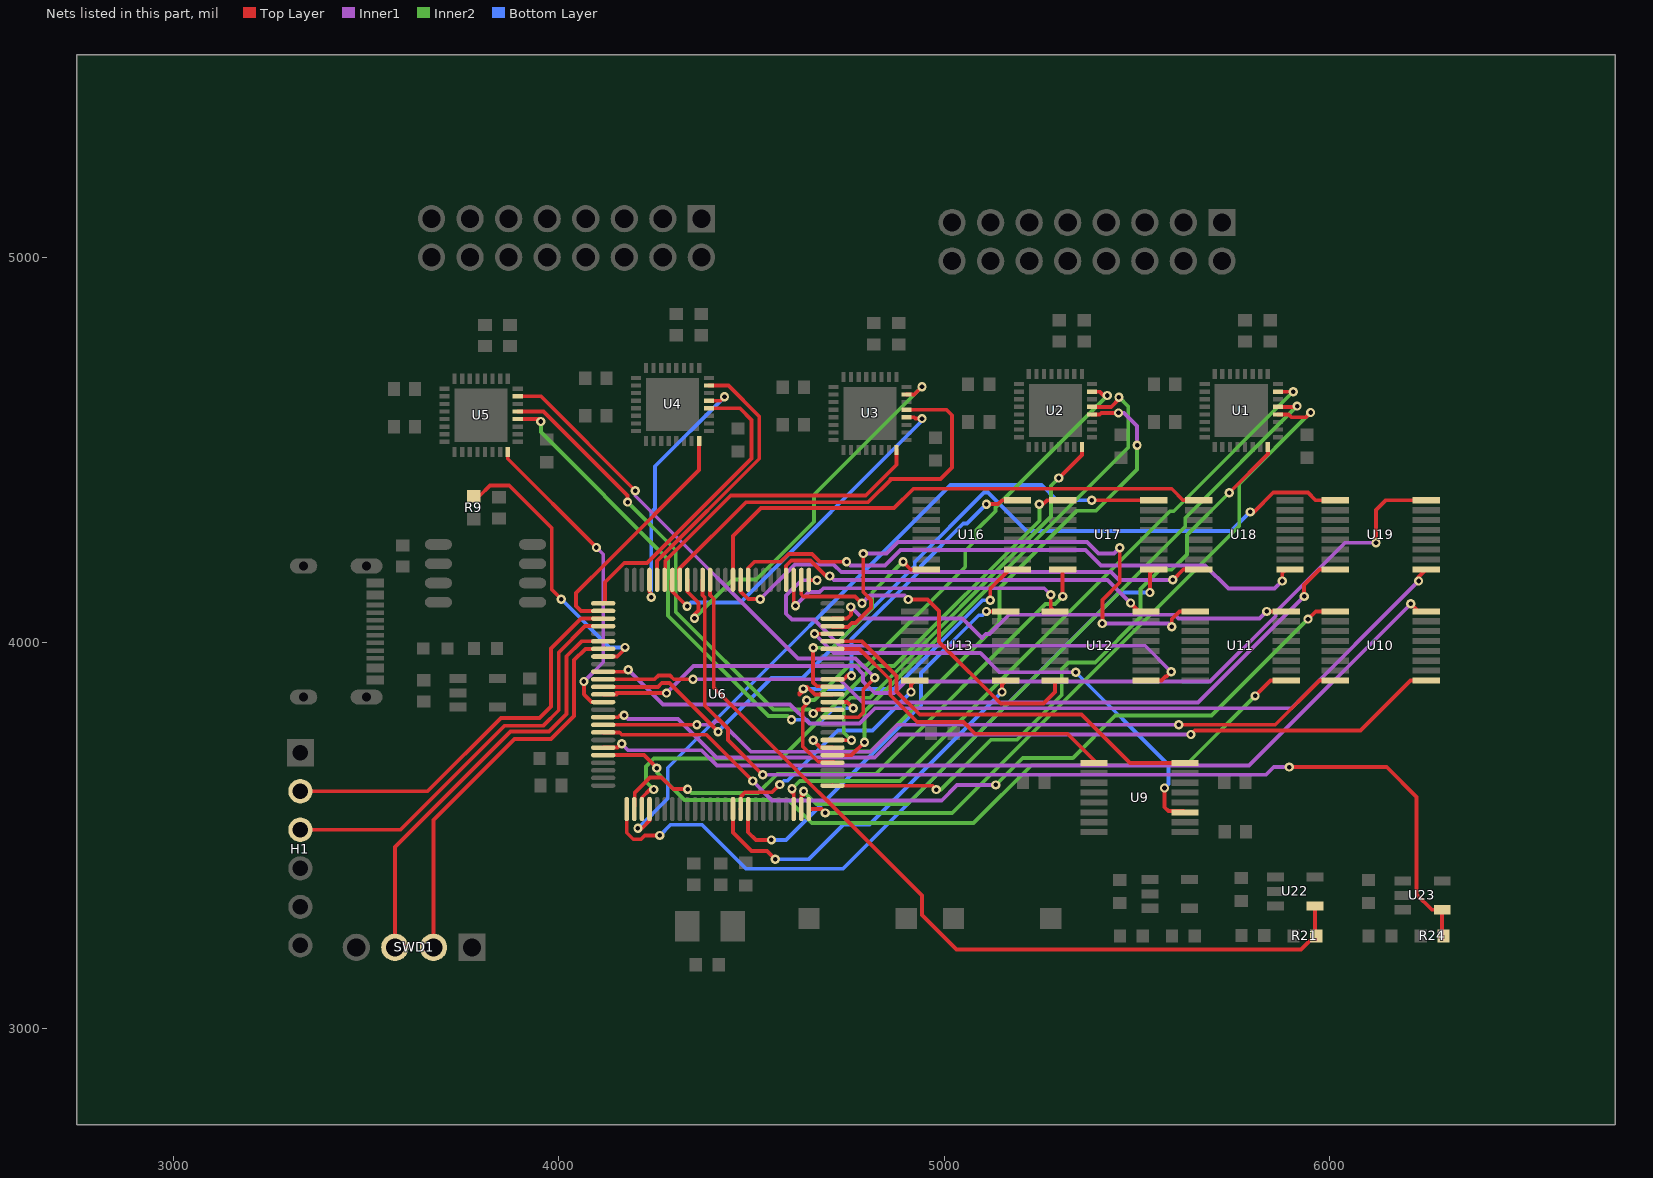
[diagram p0: the nets of this part, all layers, seen from the top]
# Altium PCB MISC49858.pcbdoc (part 3 of 3)
Units mil, origin at the board's own origin, x right, y up, seen from the top; angles counter-clockwise.
Board outline 3990 x 2775 mil, 6 copper layers (Top Layer, Inner1, Inner2, Inner3, Inner4, Bottom Layer), stack 60.565 mil thick; 79 components, 151 nets, 603 pads, 275 vias.

## Via types
v1: diameter 24.02, hole 12, Top Layer to Bottom Layer, 275 vias

## Nets (pads, with @x,y where several pads share a name; then routed paths per layer and width w, separated by ;. In a path a pad name is that pad's centre, name@x,y a point inside that pad or via, vN(x,y) a via of type N, cw(c..) or ccw(c..) an arc to the next point about the centre after c; other vN are vias at no path point) (continued)
OUT2: R21.2 U6.64 U22.4 | length 2252.9
  Top Layer w10: U6.64@4392.85,4163.23 4391.96,4162.33 4391.96,4124.12 4401.96,4114.12 4401.96,3884.12 4941.96,3344.12 4941.96,3294.12 5031.96,3204.12 5924.66,3204.12 R21.2@5964.66,3244.12 ; U22.4@5961.19,3317.6 5961.18,3247.6 R21.2@5964.66,3244.12 ; R21.2@5964.66,3240 R21.2@5964.66,3244.12
OUT3: R24.2 U6.65 U23.4 | length 2711.2
  Top Layer w10: U6.65@4373.16,4163.23 4373.16,4123.23 4378.79,4117.6 4378.79,3837.6 4438.79,3777.6 4438.79,3747.6 v1(4528.79,3657.6) ; v1(5894.53,3677.6) 6147.4,3677.6 6224.53,3600.47 6224.53,3347.6 6264.53,3307.6 U23.4@6291.19,3307.6 6291.18,3247.6 6294.66,3244.12 R24.2@6294.66,3240
  Inner1 w10: v1(4528.79,3657.6) 5834.53,3657.6 5854.53,3677.6 v1(5894.53,3677.6)
SPI1_MISO: U1.16 U6.26 | length 1623.1
  Top Layer w9.92: U6.26@4709.77,3629.77 4719.09,3629.24 4969.09,3629.24 v1(4979.09,3619.24) ; v1(5739.09,4389.23) 5839.09,4489.23 U1.16@5839.09,4507.28
  Inner2 w9.92: v1(4979.09,3619.24) 4991.78,3619.24 5121.02,3748.48 5188.48,3748.48 5304.41,3864.41 5304.41,3931.87 5321.77,3949.24 5391.49,3949.24 5509.09,4066.84 5509.09,4139.24 5559.09,4189.23 5589.09,4189.23 5629.09,4229.23 5629.09,4279.23 v1(5739.09,4389.23)
SPI1_MOSI: U1.23 U6.23 | length 1823.6
  Top Layer w9.92: v1(4604.97,3621.28) 4604.97,3611.28 4609.38,3611.28 U6.23@4609.38,3568.75 ; U1.23@5864.97,4651.27 v1(5904.97,4651.27)
  Inner2 w9.92: v1(4604.97,3621.28) 4624.97,3641.28 4884.97,3641.28 5584.97,4341.27 5594.97,4341.27 v1(5904.97,4651.27)
SPI1_SCK: U1.20 U6.25 | length 1892.5
  Top Layer w9.92: U6.25@4648.75,3568.75 4681.49,3568.75 v1(4691.49,3558.75) ; U1.20@5864.97,4592.22 5892.78,4592.22 5900,4585 5937.74,4585 v1(5949.97,4597.23)
  Inner2 w9.92: v1(4691.49,3558.75) 5020.71,3558.75 5764.97,4303.01 5764.97,4412.23 v1(5949.97,4597.23)
SPI1_SSN: U1.21 U6.24 | length 1836.4
  Top Layer w9.92: U6.24@4629.07,3568.75 4629.07,3604.65 4634.97,3604.65 v1(4634.97,3614.65) ; U1.21@5864.97,4611.9 5913.06,4611.9 v1(5914.97,4613.81)
  Inner2 w9.92: v1(4634.97,3614.65) 4667.71,3581.91 4904.97,3581.91 5624.97,4301.9 5624.97,4323.81 v1(5914.97,4613.81)
SPI2_MISO: U2.16 U6.32 | length 1104.3
  Top Layer w9.92: U6.32@4709.77,3747.88 4709.18,3747.29 v1(4759.18,3747.29) ; v1(5296.98,4427.29) 5356.98,4487.29 U2.16@5356.98,4507.28
  Inner2 w9.92: v1(4759.18,3747.29) 4739.18,3767.29 4739.18,3839.48 4756.99,3857.29 4806.99,3857.29 5276.98,4327.29 5276.98,4407.29 v1(5296.98,4427.29)
SPI2_MOSI: U2.23 U6.29 | length 1420.3
  Top Layer w9.92: v1(4642.86,3851.28) 4642.86,3841.28 4632.86,3831.28 4632.86,3731.28 4672.86,3691.28 4712.86,3691.28 U6.29@4709.77,3688.82 ; U2.23@5382.86,4651.27 5402.86,4651.27 5412.86,4641.27 v1(5422.86,4641.27)
  Inner2 w9.92: v1(4642.86,3851.28) 4662.86,3851.28 4752.86,3941.28 4798.45,3941.28 5054.17,4197 5054.17,4238.74 5083.86,4268.43 5083.86,4292.27 5132.86,4341.27 5132.86,4351.27 v1(5422.86,4641.27)
SPI2_SCK: U2.20 U6.31 | length 1511.2
  Top Layer w9.92: v1(4659.77,3747.24) 4678.82,3728.19 U6.31@4709.77,3728.19 ; U2.20@5382.86,4592.22 5402.86,4592.23 5406.83,4596.19 v1(5451.62,4596.19)
  Inner1 w9.92: v1(5451.62,4596.19) 5465.65,4596.19 5500,4561.84 v1(5500,4512.08)
  Inner2 w9.92: v1(4659.77,3747.24) 4688.82,3718.19 4808.82,3718.19 5142.86,4052.23 5142.86,4142.23 5342.86,4342.23 5392.86,4342.23 5500,4449.36 v1(5500,4512.08)
SPI2_SSN: U2.21 U6.30 | length 1369
  Top Layer w9.92: U6.30@4709.77,3708.51 4759.47,3708.51 v1(4792.86,3741.91) ; U2.21@5382.86,4611.9 5432.86,4611.9 5452.86,4631.9 v1(5452.86,4637.08)
  Inner2 w9.92: v1(4792.86,3741.91) 4792.86,3821.91 5477.05,4506.09 5477.05,4612.9 v1(5452.86,4637.08)
SPI3_MISO: U3.16 U6.70 | length 790.4
  Top Layer w9.92: U6.70@4274.73,4163.23 4276.26,4171.85 4276.26,4211.85 4446.26,4381.85 4796.26,4381.85 4876.26,4461.85 U3.16@4876.26,4499.9
SPI3_MOSI: U3.23 U6.67 | length 1043
  Top Layer w9.92: U6.67@4333.79,4163.23 4333.79,4132.24 4362.14,4103.89 4362.14,4083.89 4352.14,4073.89 v1(4352.14,4063.89) ; U3.23@4902.14,4643.89 4922.14,4643.89 v1(4942.14,4663.89)
  Inner2 w9.92: v1(4352.14,4063.89) 4452.14,4163.89 4512.14,4163.89 4662.14,4313.89 4662.14,4383.89 v1(4942.14,4663.89)
SPI3_SCK: U3.20 U6.69 | length 941.3
  Top Layer w9.92: U6.69@4294.42,4163.23 4292.81,4161.61 4292.81,4134.84 v1(4332.81,4094.84) ; U3.20@4902.14,4584.84 4922.14,4584.84 4925.57,4581.41 v1(4942.14,4581.41)
  Bottom Layer w9.92: v1(4332.81,4094.84) 4342.81,4104.84 4471.29,4104.84 4942.14,4575.69 v1(4942.14,4581.41)
SPI3_SSN: U3.21 U6.68 | length 1107.4
  Top Layer w9.92: U6.68@4314.1,4163.23 4312.14,4165.19 4312.14,4191.26 4485.4,4364.52 4802.14,4364.52 4862.62,4425 ; 4860,4425 4862.62,4425 ; U3.21@4902.14,4604.52 5005.48,4604.52 5020,4590 5020,4455 4990,4425 4862.62,4425
SPI4_MISO: U4.16 U6.77 | length 635.9
  Top Layer w9.92: 4130.33,4214.12 4364.12,4447.91 U4.16@4364.12,4523.28
  Top Layer w10: U6.77@4115.29,4082.53 4057.47,4082.53 4045,4095 4045,4128.79 4130.33,4214.12
SPI4_MOSI: U4.23 U6.71 | length 696.9
  Top Layer w9.92: U6.71@4255.05,4163.23 4255.05,4212.33 4520,4477.27 4520,4587.27 4440,4667.27 U4.23@4390,4667.27
SPI4_SCK: U4.20 U6.76 | length 792.2
  Top Layer w9.92: U6.76@4115.29,4102.21 4120,4106.91 4120,4156.91 4170,4206.91 4228.68,4206.91 4500,4478.23 4500,4578.23 4470,4608.23 U4.20@4390,4608.22
SPI4_SSN: U4.21 U6.72 | length 690.1
  Top Layer w9.92: U6.72@4235.36,4163.23 4235.36,4132.54 4240,4127.9 v1(4240,4117.9) ; U4.21@4390,4627.9 4420,4627.9 v1(4430,4637.9)
  Bottom Layer w9.92: v1(4240,4117.9) 4240,4337.9 4250,4347.9 4250,4457.9 v1(4430,4637.9)
SPI5_MISO: U5.16 U6.89 | length 810.5
  Top Layer w9.92: U5.16@3867.71,4495.22 3867.71,4477.17 v1(4097.71,4247.17) ; v1(4065.29,3899.58) 4065.29,3866.31 4085.29,3846.31 U6.89@4115.29,3846.31
  Inner1 w9.92: v1(4065.29,3899.58) 4115.29,3949.58 4115.29,4229.58 v1(4097.71,4247.17)
SPI5_MOSI: U5.23 U6.35 | length 1423.6
  Top Layer w9.92: U5.23@3893.59,4639.21 3953.59,4639.21 v1(4198.58,4394.21) ; U6.35@4709.77,3806.93 4777.49,3806.93 4789.77,3819.21 4789.77,3879.21 v1(4819.77,3909.21)
  Inner1 w9.92: v1(4198.58,4394.21) 4198.58,4381.42 4620.79,3959.21 4769.77,3959.21 v1(4819.77,3909.21)
SPI5_SCK: U5.20 U6.37 | length 1376.1
  Top Layer w9.92: U5.20@3893.59,4580.16 3947.42,4580.16 v1(3953.62,4573.96) ; U6.37@4709.77,3846.31 4747.44,3846.31 v1(4763.58,3830.16)
  Inner2 w9.92: v1(3953.62,4573.96) 3953.62,4546.38 4283.58,4216.42 4283.58,4070.16 4543.58,3810.16 4593.58,3810.16 v1(4603.58,3800.16)
  Bottom Layer w9.92: v1(4603.58,3800.16) 4643.58,3800.16 4653.58,3790.16 4673.58,3790.16 4713.58,3830.16 v1(4763.58,3830.16)
SPI5_SSN: U5.21 U6.36 | length 1248.4
  Top Layer w9.92: U5.21@3893.59,4599.84 3960.5,4599.84 4178.58,4381.75 v1(4178.58,4364.84) ; v1(4660.36,3816.62) 4670.36,3826.62 U6.36@4709.77,3826.62
  Inner2 w9.92: v1(4178.58,4364.84) 4303.58,4239.84 4303.58,4079.84 4556.8,3826.62 4650.36,3826.62 v1(4660.36,3816.62)
SWCLK: SWD1.3 U6.81 | length 1109.3
  Top Layer w10: SWD1.3@3575,3210 3575,3470 3875,3770 3975,3770 4020,3815 4020,3965 4058.79,4003.79 U6.81@4115.29,4003.79
SWDIO: SWD1.2 U6.82 | length 1039.2
  Top Layer w10: SWD1.2@3675,3210 3675,3540 3885,3750 3980,3750 4040,3810 4040,3955 4069.1,3984.1 U6.82@4115.29,3984.1
T3_SEL1: U6.44 U9.1 | length 829.8
  Top Layer w10: U6.44@4709.77,3984.1 4779.77,3984.1 4859.77,3904.1 4859.77,3864.1 4929.77,3794.1 5049.77,3794.1 5079.77,3764.1 5319.77,3764.1 5389.77,3694.1 U9.1@5388.11,3688.12
T3_SEL2: U6.45 U9.16 | length 1068.7
  Top Layer w10: U6.45@4709.77,4003.79 4786.18,4003.79 4876.18,3913.79 4876.18,3873.79 4936.18,3813.79 5356.18,3813.79 5481.84,3688.12 U9.16@5624.33,3688.12
T3_SEL3: U6.46 U9.11 | length 1277.9
  Top Layer w10: v1(4663.37,4023.47) U6.46@4709.77,4023.47 ; v1(5571.03,3623.47) 5571.03,3573.47 5581.03,3563.47 5621.03,3563.47 U9.11@5624.33,3560.16
  Inner1 w10: v1(4663.37,4023.47) 4713.37,3973.47 5093.37,3973.47 5143.37,3923.47 v1(5341.03,3923.47)
  Bottom Layer w10: v1(5341.03,3923.47) 5581.03,3683.47 5581.03,3633.47 v1(5571.03,3623.47)
T11_SEL1: U6.91 U10.1 | length 2265.3
  Top Layer w10: U6.91@4115.29,3806.93 4154.19,3806.93 4159.49,3812.23 v1(4169.49,3812.23) ; v1(5639.48,3762.23) 5649.48,3772.23 6079.48,3772.23 6209.48,3902.23 U10.1@6249.98,3902.23
  Inner1 w10: v1(4169.49,3812.23) 4179.49,3802.23 4309.49,3802.23 4409.49,3702.23 4819.49,3702.23 4879.49,3762.23 v1(5639.48,3762.23)
T11_SEL2: U6.92 U10.16 | length 2012.4
  Top Layer w10: U6.92@4115.29,3787.25 4178.29,3787.25 v1(4358.29,3787.25) ; v1(5608.28,3787.25) 5858.28,3787.25 5973.26,3902.23 U10.16@6013.76,3902.23
  Inner1 w10: v1(4358.29,3787.25) 4398.29,3787.25 4408.29,3797.25 4418.29,3797.25 4498.28,3717.25 4808.28,3717.25 4878.28,3787.25 v1(5608.28,3787.25)
T11_SEL3: U6.93 U10.9 | length 2174.4
  Top Layer w10: U6.93@4115.29,3767.56 4157.08,3767.56 4163.27,3761.37 4383.27,3761.37 v1(4503.27,3641.37) ; v1(5943.26,4061.37) 5963.26,4081.37 U10.9@6013.76,4081.37
  Inner1 w10: v1(4503.27,3641.37) 4553.27,3591.37 4993.26,3591.37 5033.26,3631.37 v1(5133.26,3631.37)
  Inner2 w10: v1(5133.26,3631.37) 5203.26,3701.37 5333.26,3701.37 5443.26,3811.37 5693.26,3811.37 v1(5943.26,4061.37)
T11_SEL4: U6.95 U10.8 | length 2344.6
  Top Layer w10: U6.95@4115.29,3728.19 4153.17,3728.19 v1(4163.17,3738.19) ; v1(6209.98,4101.37) 6229.98,4081.37 U10.8@6249.98,4081.37
  Inner1 w10: v1(4163.17,3738.19) 4179.99,3721.37 4369.99,3721.37 4409.99,3681.37 5789.98,3681.37 v1(6209.98,4101.37)
T12_SEL1: U6.96 U11.1 | length 2004
  Top Layer w10: U6.96@4115.29,3708.51 4220.84,3708.51 v1(4254.4,3674.95) ; v1(5806.06,3862.23) 5846.06,3902.23 U11.1@5886.56,3902.23
  Inner2 w10: v1(4254.4,3674.95) 4254.4,3663.89 4326.06,3592.23 4596.06,3592.23 4656.06,3532.23 5076.06,3532.23 5226.06,3682.23 5626.06,3682.23 v1(5806.06,3862.23)
T12_SEL3: U6.48 U11.8 | length 1270.7
  Top Layer w10: U6.48@4709.77,4062.84 4747.53,4062.84 4757.53,4072.84 v1(4757.53,4092.84) ; v1(5836.06,4081.37) U11.8@5886.56,4081.37
  Inner1 w10: v1(4757.53,4092.84) 4787.53,4062.84 5047.53,4062.84 5097.53,4012.84 5107.53,4022.84 5117.53,4022.84 5167.53,4072.84 5597.53,4072.84 5607.53,4062.84 5817.53,4062.84 v1(5836.06,4081.37)
T12_SEL4: U6.47 U11.9 | length 1454.3
  Top Layer w10: U6.47@4709.77,4043.16 4709.84,4041.37 4749.84,4041.37 4759.84,4051.37 4769.84,4051.37 4809.84,4091.37 4809.84,4111.37 4789.84,4131.37 v1(4789.84,4231.37) ; v1(5409.84,4049.85) 5409.84,4111.37 5454.84,4156.37 v1(5454.84,4246.37) ; v1(5589.84,4041.37) 5589.84,4061.37 5609.84,4081.37 U11.9@5650.34,4081.37
  Inner1 w10: v1(4789.84,4231.37) 4849.84,4231.37 4879.84,4261.37 5369.84,4261.37 5399.84,4231.37 5439.84,4231.37 v1(5454.84,4246.37) ; v1(5409.84,4049.85) 5581.37,4049.85 v1(5589.84,4041.37)
T13_SEL1: U6.51 U12.1 | length 1301
  Top Layer w10: U6.51@4648.75,4163.23 4649.75,4162.23 v1(4669.75,4162.23) ; U12.1@5523.14,3902.23 5563.65,3902.23 5573.65,3912.23 5576.17,3912.23 v1(5588.65,3924.7)
  Inner1 w10: v1(4669.75,4162.23) 4629.75,4162.23 4589.75,4122.23 4589.75,4075.25 4604.7,4060.3 4661.68,4060.3 4729.75,3992.23 5521.12,3992.23 v1(5588.65,3924.7)
T13_SEL2: U6.52 U12.16 | length 918.7
  Top Layer w10: U6.52@4629.07,4163.23 4629.07,4125.93 4635,4120 4768.65,4120 v1(4786.43,4102.23) ; v1(4906.43,4112.23) 4956.43,4112.23 4986.43,4082.23 4986.43,4002.23 5146.43,3842.23 5257.23,3842.23 5286.93,3871.93 U12.16@5286.92,3902.23
  Inner1 w10: v1(4786.43,4102.23) 4806.43,4122.23 4896.43,4122.23 v1(4906.43,4112.23)
T13_SEL3: U6.53 U12.9 | length 804.3
  Top Layer w10: U6.53@4609.38,4163.23 4609.38,4101.16 v1(4614.17,4096.37) ; v1(5275.96,4124.7) 5275.96,4091.84 5286.43,4081.37 U12.9@5286.92,4081.37
  Inner1 w10: v1(4614.17,4096.37) 4649.17,4131.37 4676.43,4131.37 4686.43,4141.37 5259.29,4141.37 v1(5275.96,4124.7)
T13_SEL4: U6.54 U12.8 | length 1030.2
  Top Layer w9.92: v1(5483.15,4103.23) 5505,4081.37 U12.8@5523.14,4081.37
  Top Layer w10: U6.54@4589.7,4163.23 4589.7,4199.78 4603.15,4213.23 4653.15,4213.23 4693.15,4173.23 v1(4703.15,4173.23)
  Inner1 w10: v1(4703.15,4173.23) 4713.15,4163.23 5423.15,4163.23 v1(5483.15,4103.23)
T14_SEL1: U6.15 U13.1 | length 1001
  Top Layer w10: U6.15@4451.9,3568.75 4451.9,3507.92 4499.82,3460 4539.99,3460 v1(4561.25,3438.75) ; v1(5149.72,3872.23) 5149.72,3892.23 U13.1@5159.72,3902.23
  Bottom Layer w10: v1(4561.25,3438.75) 4648.75,3438.75 4738.75,3528.75 4806.25,3528.75 v1(5149.72,3872.23)
T14_SEL2: U6.16 U13.16 | length 620
  Top Layer w10: U6.16@4471.59,3568.75 4473.51,3572.23 4473.51,3602.23 4483.51,3612.23 4553.51,3612.23 v1(4573.51,3632.23) ; v1(4913.5,3872.23) 4913.5,3892.23 U13.16@4923.5,3902.23
  Bottom Layer w10: v1(4573.51,3632.23) 4583.51,3642.23 4593.51,3642.23 4723.51,3772.23 4813.51,3772.23 v1(4913.5,3872.23)
T14_SEL4: U6.17 U13.8 | length 1030.5
  Top Layer w10: U6.17@4491.27,3568.75 4491.27,3508.73 4511.25,3488.75 v1(4551.6,3488.75) ; v1(5109.22,4081.37) U13.8@5159.72,4081.37
  Bottom Layer w10: v1(4551.6,3488.75) 4588.97,3488.75 4939.23,3839 4939.23,3921.37 5089.22,4071.37 5099.22,4071.37 v1(5109.22,4081.37)
T21_SEL1: U6.85 U19.1 | length 2366.4
  Top Layer w10: U6.85@4115.29,3925.05 4174.69,3925.05 v1(4179.99,3930.34) ; v1(6229.98,4160.34) 6229.98,4170.34 U19.1@6249.98,4190.34
  Inner1 w10: v1(4179.99,3930.34) 4269.99,3840.34 4599.99,3840.34 4649.99,3790.34 4779.99,3790.34 4819.99,3830.34 5899.98,3830.34 v1(6229.98,4160.34)
T21_SEL2: U6.86 U19.16 | length 2092.1
  Top Layer w10: U6.86@4115.29,3905.36 4248.28,3905.36 4258.28,3915.36 4288.28,3915.36 4298.28,3905.36 v1(4348.28,3905.36) ; v1(5933.26,4120.34) 5933.26,4150.34 5973.26,4190.34 U19.16@6013.76,4190.34
  Inner1 w10: v1(4348.28,3905.36) 4728.28,3905.36 4788.28,3845.36 5658.28,3845.36 v1(5933.26,4120.34)
T21_SEL3: U6.87 U19.9 | length 2308.7
  Top Layer w10: U6.87@4115.29,3885.68 4257.07,3885.68 4267.07,3895.68 4287.07,3895.68 v1(4413.27,3769.48) ; v1(5793.26,4339.48) 5803.26,4339.48 5853.26,4389.48 5943.26,4389.48 5963.26,4369.48 U19.9@6013.76,4369.48
  Bottom Layer w10: v1(4413.27,3769.48) 4553.27,3909.48 4633.27,3909.48 4923.26,4199.48 4923.26,4209.48 5103.26,4389.48 5113.26,4389.48 5213.26,4289.48 5743.26,4289.48 v1(5793.26,4339.48)
T21_SEL4: U6.88 U19.8 | length 2470.6
  Top Layer w10: U6.88@4115.29,3865.99 4149.49,3865.99 4149.49,3869.48 v1(4279.49,3869.48) ; v1(6119.48,4259.48) 6119.48,4344.48 6144.48,4369.48 U19.8@6249.98,4369.48
  Inner1 w10: v1(4279.49,3869.48) 4349.49,3939.48 4769.49,3939.48 4789.49,3919.48 4789.49,3899.48 4819.49,3869.48 4869.49,3869.48 4899.48,3899.48 5689.48,3899.48 5859.48,4069.48 5859.48,4079.48 6039.48,4259.48 v1(6119.48,4259.48)
T22_SEL1: U6.59 U18.1 | length 1553.5
  Top Layer w10: U6.59@4491.27,4163.23 4491.27,4193.23 4508.39,4210.34 4576.56,4210.34 4596.56,4230.34 4656.56,4230.34 4676.56,4210.34 v1(4746.56,4210.34) ; v1(5876.56,4160.34) 5876.56,4180.34 5886.56,4190.34 U18.1@5896.56,4190.34
  Inner1 w10: v1(4746.56,4210.34) 4756.56,4200.34 4846.56,4200.34 4886.56,4240.34 5366.56,4240.34 5406.56,4200.34 5676.56,4200.34 5736.56,4140.34 5856.56,4140.34 v1(5876.56,4160.34)
T22_SEL2: U6.60 U18.16 | length 1292.1
  Top Layer w10: U6.60@4471.59,4163.23 4471.59,4133.23 4491.59,4113.23 v1(4522.73,4113.23) ; v1(5592.73,4163.23) 5619.84,4190.34 U18.16@5660.34,4190.34
  Inner1 w10: v1(4522.73,4113.23) 4612.73,4203.23 4712.73,4203.23 4732.73,4183.23 5432.73,4183.23 5452.73,4163.23 v1(5592.73,4163.23)
T22_SEL3: U6.61 U18.9 | length 1385.3
  Top Layer w10: U6.61@4451.9,4163.23 4451.9,4276.9 4524.48,4349.48 4869.84,4349.48 4919.84,4399.48 5589.84,4399.48 5619.84,4369.48 U18.9@5660.34,4369.48
T23_SEL1: U6.1 U17.1 | length 1849
  Top Layer w10: U6.1@4176.31,3568.75 4176.31,3507.18 4193.15,3490.34 4213.15,3490.34 4223.15,3500.34 v1(4262.25,3500.34) ; v1(5533.15,4130.34) 5533.15,4180.34 U17.1@5543.14,4190.34
  Bottom Layer w10: v1(4262.25,3500.34) 4289.9,3527.99 4372.01,3527.99 4485.98,3414.02 4736.82,3414.02 5453.15,4130.34 v1(5533.15,4130.34)
T23_SEL2: U6.2 U17.16 | length 1466
  Top Layer w10: U6.2@4195.99,3568.75 4196.93,3580.34 4196.93,3610.34 4236.93,3650.34 4266.93,3650.34 4296.93,3620.34 v1(4334.17,3620.34) ; v1(5306.93,4120.34) U17.16@5306.92,4190.34
  Inner2 w10: v1(4334.17,3620.34) 4344.17,3610.34 4516.93,3610.34 4566.93,3660.34 4822.83,3660.34 5262.83,4100.34 5286.93,4100.34 v1(5306.93,4120.34)
T23_SEL3: U6.3 U17.9 | length 1528.8
  Top Layer w10: U6.3@4215.68,3568.75 4216.43,3579.48 4216.43,3599.48 4236.43,3619.48 v1(4246.43,3619.48) ; v1(5246.43,4359.48) 5256.43,4359.48 5266.43,4369.48 U17.9@5306.92,4369.48
  Inner2 w10: v1(4246.43,3619.48) 4226.43,3639.48 4226.43,3679.48 4246.43,3699.48 4576.43,3699.48 4816.43,3939.48 4869.42,3939.48 5246.43,4316.49 v1(5246.43,4359.48)
T23_SEL4: U6.4 U17.8 | length 1838.5
  Top Layer w10: v1(4205.36,3518.75) 4215.36,3518.75 4235.36,3538.75 U6.4@4235.36,3568.75 ; v1(5382.65,4369.48) 5502.65,4369.48 U17.8@5543.14,4369.48
  Bottom Layer w10: v1(4205.36,3518.75) 4282.65,3596.03 4282.65,3676.03 5016.1,4409.48 5252.65,4409.48 5292.65,4369.48 v1(5382.65,4369.48)
T24_SEL1: U6.38 U16.1 | length 822.3
  Top Layer w10: v1(4634.13,3880.34) 4624.13,3870.34 4624.13,3865.99 4644.13,3885.99 4664.13,3865.99 U6.38@4709.77,3865.99 ; v1(5119.22,4110.34) 5119.22,4140.34 5169.22,4190.34 U16.1@5189.72,4190.34
  Bottom Layer w10: v1(4634.13,3880.34) 4869.23,3880.34 5099.22,4110.34 v1(5119.22,4110.34)
T24_SEL2: U6.39 U16.16 | length 562.2
  Top Layer w10: v1(4659.77,3987.11) 4659.77,3897.11 4669.77,3887.11 4699.77,3887.11 U6.39@4709.77,3885.68 ; v1(4893,4210.34) 4913,4190.34 U16.16@4953.5,4190.34
  Inner2 w10: v1(4659.77,3987.11) 4709.77,3987.11 4813,4090.34 4813,4130.34 v1(4893,4210.34)
T24_SEL4: U6.40 U16.8 | length 733.8
  Top Layer w10: U6.40@4709.77,3905.36 4719.23,3904.81 4739.23,3904.81 4749.23,3914.81 v1(4759.23,3914.81) ; v1(5109.22,4359.48) 5139.22,4359.48 5149.22,4369.48 U16.8@5189.72,4369.48
  Bottom Layer w10: v1(4759.23,3914.81) 4759.23,4009.48 4939.23,4189.48 4939.23,4199.48 5049.22,4309.48 5059.22,4309.48 v1(5109.22,4359.48)
UART4-RX: H1.3 U6.79 | length 1091.9
  Top Layer w10: H1.3@3330,3515 3590,3515 3860,3785 3960,3785 4000,3825 4000,3975 4068.16,4043.16 U6.79@4115.29,4043.16
UART4-TX: H1.2 U6.78 | length 1058.7
  Top Layer w10: H1.2@3330,3615 3660,3615 3850,3805 3950,3805 3980,3835 3980,3985 4057.84,4062.84 U6.78@4115.29,4062.84
USART1_TX: R9.2 U6.83 | length 739.6
  Top Layer w10: R9.2@3779.66,4380 3793.74,4380 3821.7,4407.96 3871.7,4407.96 3981.7,4297.96 3981.7,4137.96 v1(4006.7,4112.96) ; U6.83@4115.29,3964.42 4151.7,3964.42 4171.7,3984.42 v1(4171.7,3987.96)
  Bottom Layer w10: v1(4006.7,4112.96) 4131.7,3987.96 v1(4171.7,3987.96)
pads on no net: H1.1 H1.6 U1.4 U1.5 U1.7 U1.8 U1.9 U1.11 U1.12 U1.13 U1.14 U1.15 U1.22 U1.33 U2.4 U2.5 U2.7 U2.8 U2.9 U2.11 U2.12 U2.13 U2.14 U2.15 U2.22 U2.33 U3.4 U3.5 U3.7 U3.8 U3.9 U3.11 U3.12 U3.13 U3.14 U3.15 U3.22 U3.33 U4.4 U4.5 U4.7 U4.8 U4.9 U4.11 U4.12 U4.13 U4.14 U4.15 U4.22 U4.33 U5.4 U5.5 U5.7 U5.8 U5.9 U5.11 U5.12 U5.13 U5.14 U5.15 U5.22 U5.33 U6.7 U6.8 U6.9 U6.73 U7.4 U7.6 U8.4 U9.4 U9.6 U9.7 U9.8 U9.12 U10.4 U10.12 U11.4 U11.12 U11.15 U11.16 U12.4 U12.12 U13.4 U13.9 U13.10 U13.11 U13.12 U16.4 U16.9 U16.10 U16.11 U16.12 U17.4 U17.12 U18.4 U18.6 U18.7 U18.8 U18.12 U19.4 U19.12 USB1.1 USB1.2 USB1.3 USB1.4 USB1.A5 USB1.A8 USB1.B5 USB1.B8

## Polygon pours and split planes (outlines as drawn)
GND on Bottom Layer (solid, remove dead copper, pour order 2): 3000,5275 3000,3000 6490,3000 6490,5275
GND on Top Layer (solid, remove dead copper, pour order 0): 3105,5225 3105,3005 6445,3005 6445,5225

## Keep-outs
Board Outline Layer:
  lines w10: 3235,3115 3235,5150 6365,5150 6365,3115 3235,3115